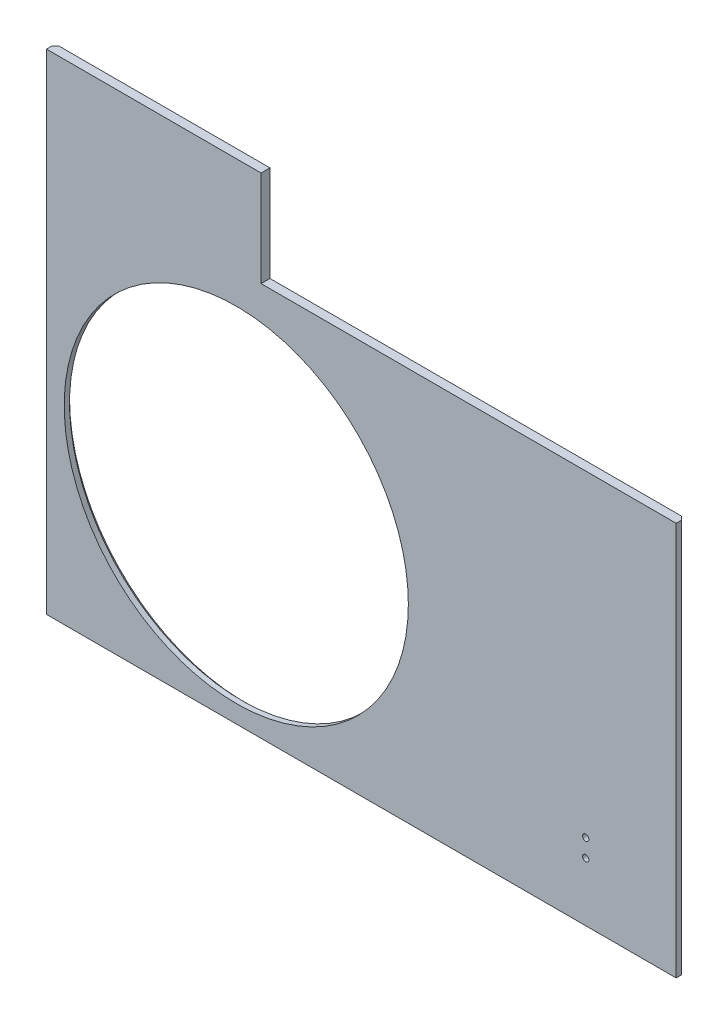
SolidWorks part; units mm, degrees
material "Q235"
ref_plane "Front Plane" through (0, 0, 0) normal (0, 0, 1) x (1, 0, 0)
ref_plane "Top Plane" through (0, 0, 0) normal (0, 1, 0) x (1, 0, 0)
ref_plane "Right Plane" through (0, 0, 0) normal (1, 0, 0) x (0, 0, -1)
sketch "Sketch1" plane through (0, 0, 0) normal (0, 0, 1) x (1, 0, 0)
  line L0 (0, 0) -> (1775, 0)
  line L1 (1775, 0) -> (1775, 1110)
  line L2 (1775, 1110) -> (605, 1110)
  line L3 (605, 1110) -> (605, 1380)
  line L4 (605, 1380) -> (0, 1380)
  line L5 (0, 1380) -> (0, 0)
  circle A1 centre (535, 535) radius 485
  dimension "D5" = 535
  dimension "D6" = 970
  dimension "D7" = 535
  dimension "D1" = 1380
  dimension "D2" = 1775
  dimension "D3" = 605
  dimension "D4" = 1110
extrude "Boss-Extrude1" add sketch "Sketch1" along normal blind 25
chamfer "Chamfer1" distance 10 angle 45 4 edges at (1020, 535, 0) (0, 690, 0) (1775, 555, 0) (887.5, 0, 0)
hole_wizard "M20 Threaded hole1" positions "3DSketch1" profile "Sketch2" tap size "M20" standard "GB" end condition through all
sketch3d "3DSketch1"
  point P0 (1520, 215, 0)
  point P2 (1520, 165, 0)
  dimension "D1" = 165
  dimension "D2" = 255
  dimension "D3" = 50
sketch "Sketch2" plane through (1520, 215, 0) normal (1, 0, 0) x (0, 1, 0)
  line L0 (0, 0) -> (0, 25)
  line L1 (0, 25) -> (8.75, 25)
  line L2 (8.75, 25) -> (8.75, 0)
  line L5 (8.75, 0) -> (0, 0)
  line L11 (0, -6.35) -> (0, 107.95) construction
  dimension "通孔螺纹孔钻头直径" = 17.5
  dimension "通孔螺纹孔钻头深度" = 25
cosmetic thread "孔螺蚊线1" parameters "D2"=20
cosmetic thread "孔螺蚊线2" parameters "D2"=20
